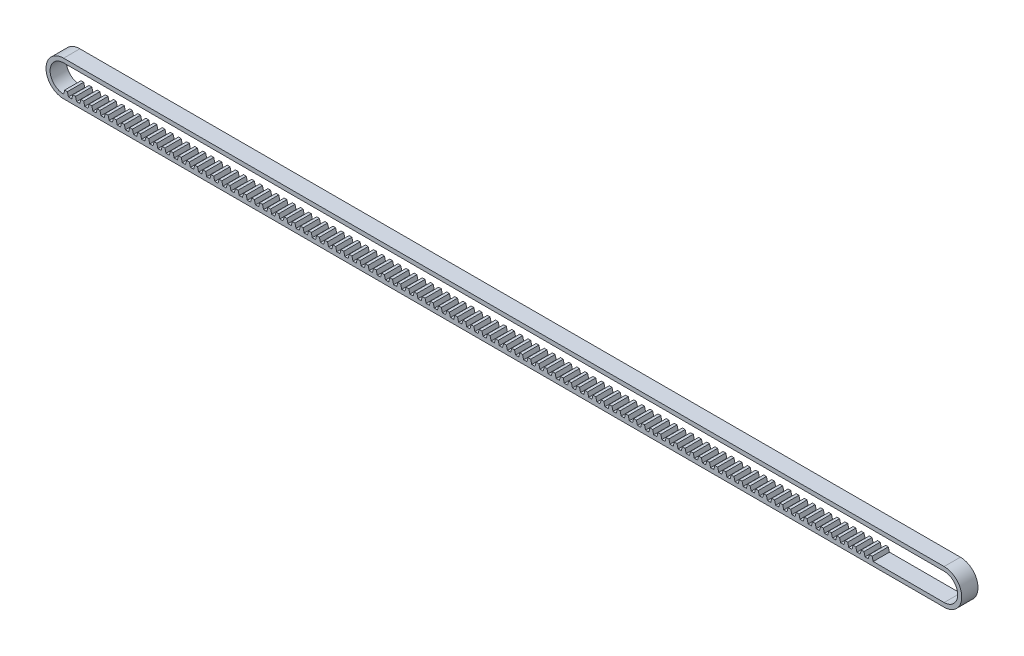
from build123d import *

# Parameters (mm, degrees)
BOSS_EXTRUDE1_DEPTH = 6
BOSS_EXTRUDE2_DEPTH = 6
LPATTERN1_COUNT     = 100
LPATTERN1_PITCH     = 3


with BuildPart() as part:
    # Sketch1 → Boss-Extrude1 (new body)
    with BuildSketch(Plane.XY):
        with BuildLine():
            Line((-162.5, -6.5), (162.5, -6.5))
            ThreePointArc((162.5, -6.5), (169, 0), (162.5, 6.5))
            Line((162.5, 6.5), (-162.5, 6.5))
            ThreePointArc((-162.5, 6.5), (-169, 0), (-162.5, -6.5))
        make_face()
        with BuildLine():
            Line((-162.5, -5), (162.5, -5))
            ThreePointArc((162.5, -5), (167.5, 0), (162.5, 5))
            Line((162.5, 5), (-162.5, 5))
            ThreePointArc((-162.5, 5), (-167.5, 0), (-162.5, -5))
        make_face(mode=Mode.SUBTRACT)
    extrude(amount=BOSS_EXTRUDE1_DEPTH)

    # Sketch2 → Boss-Extrude2 (add)
    with BuildSketch(Plane.XY.offset(6)):
        Polygon((-162.5, -5), (-162.098076211, -3.5), (-161.098076211, -3.5), (-160.696152423, -5), align=None)
    boss_extrude2 = extrude(amount=-BOSS_EXTRUDE2_DEPTH)

    # LPattern1: Boss-Extrude2 ×100
    with Locations(*[(i * LPATTERN1_PITCH, 0, 0) for i in range(1, LPATTERN1_COUNT)]):
        add(boss_extrude2)


solid = part.part
